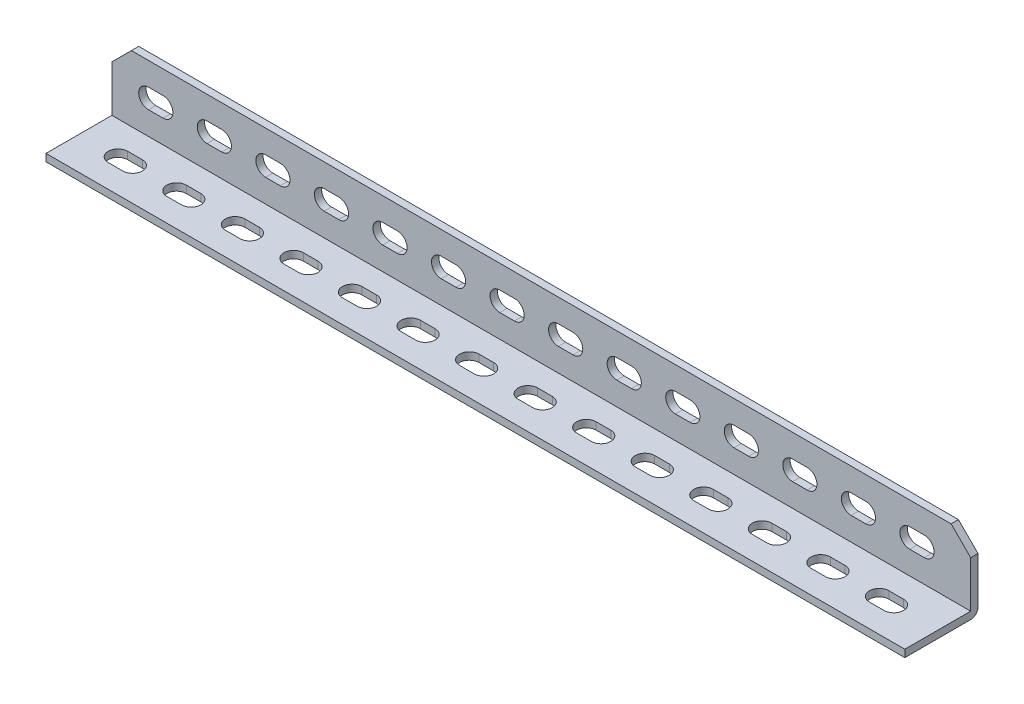
from build123d import *

# Parameters (mm, degrees)
SKETCH1_W           = 352
SKETCH1_H           = 27
BOSS_EXTRUDE1_DEPTH = 3
SKETCH3_W           = 352
SKETCH3_H           = 30
BOSS_EXTRUDE2_DEPTH = 3
FILLET1_R           = 3
CUT_EXTRUDE1_DEPTH  = 3
CUT_EXTRUDE2_DEPTH  = 3
CUT_EXTRUDE4_DEPTH  = 3


with BuildPart() as part:
    # Sketch1 → Boss-Extrude1 (new body)
    with BuildSketch(Plane.XY):
        with Locations((106.75597726, -15.498286177)):
            Rectangle(SKETCH1_W, SKETCH1_H)
    extrude(amount=BOSS_EXTRUDE1_DEPTH)

    # Sketch3 → Boss-Extrude2 (add)
    with BuildSketch(Plane.XZ.offset(28.998286177)):
        with Locations((106.75597726, 15)):
            Rectangle(SKETCH3_W, SKETCH3_H)
    extrude(amount=BOSS_EXTRUDE2_DEPTH)

    # Fillet1
    fillet1_edges = [part.edges().sort_by_distance(p)[0] for p in [
        (106.75597726, -31.998286177, 0),
    ]]
    fillet(fillet1_edges, radius=FILLET1_R)

    # Sketch4 → Cut-Extrude1 (cut)
    with BuildSketch(Plane(origin=(0, -28.998286177, 0), x_dir=(1, 0, 0), z_dir=(0, 1, 0))):
        with BuildLine():
            Line((-53.24402274, -12.5), (-47.24402274, -12.5))
            ThreePointArc((-47.24402274, -12.5), (-43.24402274, -16.5), (-47.24402274, -20.5))
            Line((-47.24402274, -20.5), (-53.24402274, -20.5))
            ThreePointArc((-53.24402274, -20.5), (-57.24402274, -16.5), (-53.24402274, -12.5))
        make_face()
        with BuildLine():
            Line((-29.24402274, -12.5), (-23.24402274, -12.5))
            ThreePointArc((-23.24402274, -12.5), (-19.24402274, -16.5), (-23.24402274, -20.5))
            Line((-23.24402274, -20.5), (-29.24402274, -20.5))
            ThreePointArc((-29.24402274, -20.5), (-33.24402274, -16.5), (-29.24402274, -12.5))
        make_face()
        with BuildLine():
            Line((-5.24402274, -12.5), (0.75597726, -12.5))
            ThreePointArc((0.75597726, -12.5), (4.75597726, -16.5), (0.75597726, -20.5))
            Line((0.75597726, -20.5), (-5.24402274, -20.5))
            ThreePointArc((-5.24402274, -20.5), (-9.24402274, -16.5), (-5.24402274, -12.5))
        make_face()
        with BuildLine():
            Line((18.75597726, -12.5), (24.75597726, -12.5))
            ThreePointArc((24.75597726, -12.5), (28.75597726, -16.5), (24.75597726, -20.5))
            Line((24.75597726, -20.5), (18.75597726, -20.5))
            ThreePointArc((18.75597726, -20.5), (14.75597726, -16.5), (18.75597726, -12.5))
        make_face()
        with BuildLine():
            Line((42.75597726, -12.5), (48.75597726, -12.5))
            ThreePointArc((48.75597726, -12.5), (52.75597726, -16.5), (48.75597726, -20.5))
            Line((48.75597726, -20.5), (42.75597726, -20.5))
            ThreePointArc((42.75597726, -20.5), (38.75597726, -16.5), (42.75597726, -12.5))
        make_face()
        with BuildLine():
            Line((66.75597726, -12.5), (72.75597726, -12.5))
            ThreePointArc((72.75597726, -12.5), (76.75597726, -16.5), (72.75597726, -20.5))
            Line((72.75597726, -20.5), (66.75597726, -20.5))
            ThreePointArc((66.75597726, -20.5), (62.75597726, -16.5), (66.75597726, -12.5))
        make_face()
        with BuildLine():
            Line((90.75597726, -12.5), (96.75597726, -12.5))
            ThreePointArc((96.75597726, -12.5), (100.75597726, -16.5), (96.75597726, -20.5))
            Line((96.75597726, -20.5), (90.75597726, -20.5))
            ThreePointArc((90.75597726, -20.5), (86.75597726, -16.5), (90.75597726, -12.5))
        make_face()
        with BuildLine():
            Line((114.75597726, -12.5), (120.75597726, -12.5))
            ThreePointArc((120.75597726, -12.5), (124.75597726, -16.5), (120.75597726, -20.5))
            Line((120.75597726, -20.5), (114.75597726, -20.5))
            ThreePointArc((114.75597726, -20.5), (110.75597726, -16.5), (114.75597726, -12.5))
        make_face()
        with BuildLine():
            Line((138.75597726, -12.5), (144.75597726, -12.5))
            ThreePointArc((144.75597726, -12.5), (148.75597726, -16.5), (144.75597726, -20.5))
            Line((144.75597726, -20.5), (138.75597726, -20.5))
            ThreePointArc((138.75597726, -20.5), (134.75597726, -16.5), (138.75597726, -12.5))
        make_face()
        with BuildLine():
            Line((162.75597726, -12.5), (168.75597726, -12.5))
            ThreePointArc((168.75597726, -12.5), (172.75597726, -16.5), (168.75597726, -20.5))
            Line((168.75597726, -20.5), (162.75597726, -20.5))
            ThreePointArc((162.75597726, -20.5), (158.75597726, -16.5), (162.75597726, -12.5))
        make_face()
        with BuildLine():
            Line((186.75597726, -12.5), (192.75597726, -12.5))
            ThreePointArc((192.75597726, -12.5), (196.75597726, -16.5), (192.75597726, -20.5))
            Line((192.75597726, -20.5), (186.75597726, -20.5))
            ThreePointArc((186.75597726, -20.5), (182.75597726, -16.5), (186.75597726, -12.5))
        make_face()
        with BuildLine():
            Line((210.75597726, -12.5), (216.75597726, -12.5))
            ThreePointArc((216.75597726, -12.5), (220.75597726, -16.5), (216.75597726, -20.5))
            Line((216.75597726, -20.5), (210.75597726, -20.5))
            ThreePointArc((210.75597726, -20.5), (206.75597726, -16.5), (210.75597726, -12.5))
        make_face()
        with BuildLine():
            Line((234.75597726, -12.5), (240.75597726, -12.5))
            ThreePointArc((240.75597726, -12.5), (244.75597726, -16.5), (240.75597726, -20.5))
            Line((240.75597726, -20.5), (234.75597726, -20.5))
            ThreePointArc((234.75597726, -20.5), (230.75597726, -16.5), (234.75597726, -12.5))
        make_face()
        with BuildLine():
            Line((258.75597726, -12.5), (264.75597726, -12.5))
            ThreePointArc((264.75597726, -12.5), (268.75597726, -16.5), (264.75597726, -20.5))
            Line((264.75597726, -20.5), (258.75597726, -20.5))
            ThreePointArc((258.75597726, -20.5), (254.75597726, -16.5), (258.75597726, -12.5))
        make_face()
    extrude(amount=-CUT_EXTRUDE1_DEPTH, mode=Mode.SUBTRACT)

    # Sketch5 → Cut-Extrude2 (cut)
    with BuildSketch(Plane.XY.offset(3)):
        with BuildLine():
            Line((-54.24402274, -11.498286177), (-48.24402274, -11.498286177))
            ThreePointArc((-48.24402274, -11.498286177), (-44.24402274, -15.498286177), (-48.24402274, -19.498286177))
            Line((-48.24402274, -19.498286177), (-54.24402274, -19.498286177))
            ThreePointArc((-54.24402274, -19.498286177), (-58.24402274, -15.498286177), (-54.24402274, -11.498286177))
        make_face()
        with BuildLine():
            Line((-30.24402274, -11.498286177), (-24.24402274, -11.498286177))
            ThreePointArc((-24.24402274, -11.498286177), (-20.24402274, -15.498286177), (-24.24402274, -19.498286177))
            Line((-24.24402274, -19.498286177), (-30.24402274, -19.498286177))
            ThreePointArc((-30.24402274, -19.498286177), (-34.24402274, -15.498286177), (-30.24402274, -11.498286177))
        make_face()
        with BuildLine():
            Line((-6.24402274, -11.498286177), (-0.24402274, -11.498286177))
            ThreePointArc((-0.24402274, -11.498286177), (3.75597726, -15.498286177), (-0.24402274, -19.498286177))
            Line((-0.24402274, -19.498286177), (-6.24402274, -19.498286177))
            ThreePointArc((-6.24402274, -19.498286177), (-10.24402274, -15.498286177), (-6.24402274, -11.498286177))
        make_face()
        with BuildLine():
            Line((17.75597726, -11.498286177), (23.75597726, -11.498286177))
            ThreePointArc((23.75597726, -11.498286177), (27.75597726, -15.498286177), (23.75597726, -19.498286177))
            Line((23.75597726, -19.498286177), (17.75597726, -19.498286177))
            ThreePointArc((17.75597726, -19.498286177), (13.75597726, -15.498286177), (17.75597726, -11.498286177))
        make_face()
        with BuildLine():
            Line((41.75597726, -11.498286177), (47.75597726, -11.498286177))
            ThreePointArc((47.75597726, -11.498286177), (51.75597726, -15.498286177), (47.75597726, -19.498286177))
            Line((47.75597726, -19.498286177), (41.75597726, -19.498286177))
            ThreePointArc((41.75597726, -19.498286177), (37.75597726, -15.498286177), (41.75597726, -11.498286177))
        make_face()
        with BuildLine():
            Line((65.75597726, -11.498286177), (71.75597726, -11.498286177))
            ThreePointArc((71.75597726, -11.498286177), (75.75597726, -15.498286177), (71.75597726, -19.498286177))
            Line((71.75597726, -19.498286177), (65.75597726, -19.498286177))
            ThreePointArc((65.75597726, -19.498286177), (61.75597726, -15.498286177), (65.75597726, -11.498286177))
        make_face()
        with BuildLine():
            Line((89.75597726, -11.498286177), (95.75597726, -11.498286177))
            ThreePointArc((95.75597726, -11.498286177), (99.75597726, -15.498286177), (95.75597726, -19.498286177))
            Line((95.75597726, -19.498286177), (89.75597726, -19.498286177))
            ThreePointArc((89.75597726, -19.498286177), (85.75597726, -15.498286177), (89.75597726, -11.498286177))
        make_face()
        with BuildLine():
            Line((113.75597726, -11.498286177), (119.75597726, -11.498286177))
            ThreePointArc((119.75597726, -11.498286177), (123.75597726, -15.498286177), (119.75597726, -19.498286177))
            Line((119.75597726, -19.498286177), (113.75597726, -19.498286177))
            ThreePointArc((113.75597726, -19.498286177), (109.75597726, -15.498286177), (113.75597726, -11.498286177))
        make_face()
        with BuildLine():
            Line((137.75597726, -11.498286177), (143.75597726, -11.498286177))
            ThreePointArc((143.75597726, -11.498286177), (147.75597726, -15.498286177), (143.75597726, -19.498286177))
            Line((143.75597726, -19.498286177), (137.75597726, -19.498286177))
            ThreePointArc((137.75597726, -19.498286177), (133.75597726, -15.498286177), (137.75597726, -11.498286177))
        make_face()
        with BuildLine():
            Line((161.75597726, -11.498286177), (167.75597726, -11.498286177))
            ThreePointArc((167.75597726, -11.498286177), (171.75597726, -15.498286177), (167.75597726, -19.498286177))
            Line((167.75597726, -19.498286177), (161.75597726, -19.498286177))
            ThreePointArc((161.75597726, -19.498286177), (157.75597726, -15.498286177), (161.75597726, -11.498286177))
        make_face()
        with BuildLine():
            Line((185.75597726, -11.498286177), (191.75597726, -11.498286177))
            ThreePointArc((191.75597726, -11.498286177), (195.75597726, -15.498286177), (191.75597726, -19.498286177))
            Line((191.75597726, -19.498286177), (185.75597726, -19.498286177))
            ThreePointArc((185.75597726, -19.498286177), (181.75597726, -15.498286177), (185.75597726, -11.498286177))
        make_face()
        with BuildLine():
            Line((209.75597726, -11.498286177), (215.75597726, -11.498286177))
            ThreePointArc((215.75597726, -11.498286177), (219.75597726, -15.498286177), (215.75597726, -19.498286177))
            Line((215.75597726, -19.498286177), (209.75597726, -19.498286177))
            ThreePointArc((209.75597726, -19.498286177), (205.75597726, -15.498286177), (209.75597726, -11.498286177))
        make_face()
        with BuildLine():
            Line((233.75597726, -11.498286177), (239.75597726, -11.498286177))
            ThreePointArc((239.75597726, -11.498286177), (243.75597726, -15.498286177), (239.75597726, -19.498286177))
            Line((239.75597726, -19.498286177), (233.75597726, -19.498286177))
            ThreePointArc((233.75597726, -19.498286177), (229.75597726, -15.498286177), (233.75597726, -11.498286177))
        make_face()
        with BuildLine():
            Line((257.75597726, -11.498286177), (263.75597726, -11.498286177))
            ThreePointArc((263.75597726, -11.498286177), (267.75597726, -15.498286177), (263.75597726, -19.498286177))
            Line((263.75597726, -19.498286177), (257.75597726, -19.498286177))
            ThreePointArc((257.75597726, -19.498286177), (253.75597726, -15.498286177), (257.75597726, -11.498286177))
        make_face()
    extrude(amount=-CUT_EXTRUDE2_DEPTH, mode=Mode.SUBTRACT)

    # Sketch6 → Cut-Extrude4 (cut)
    with BuildSketch(Plane.XY.offset(3)):
        Polygon((-69.24402274, -1.998286177), (-69.24402274, -7.998286177), (-69.24402274, -9.998286177), (-61.24402274, -1.998286177), align=None)
        Polygon((274.75597726, -1.998286177), (282.75597726, -1.998286177), (282.75597726, -9.998286177), align=None)
    extrude(amount=-CUT_EXTRUDE4_DEPTH, mode=Mode.SUBTRACT)


solid = part.part
